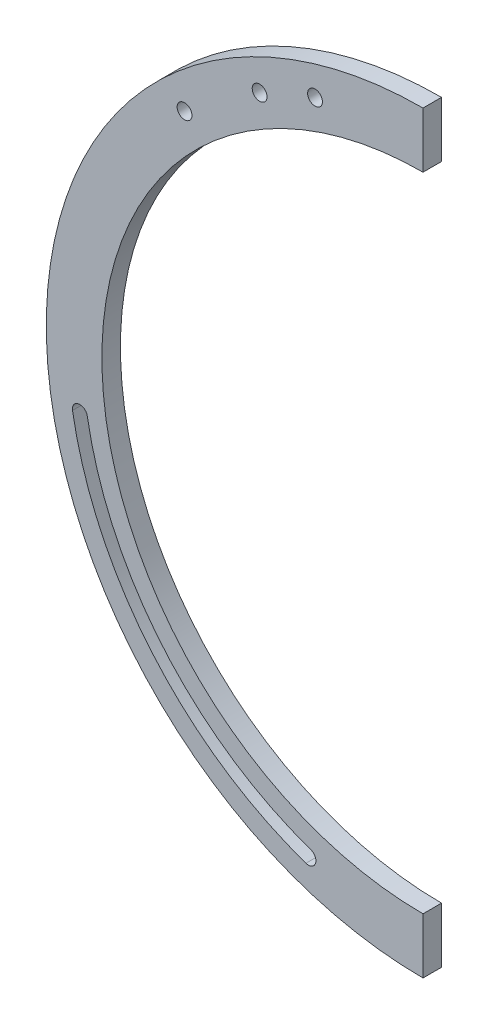
from build123d import *

# Parameters (mm, degrees)
SKETCH1_R               = 203.294925519
SKETCH1_R_2             = 173.294925519
BOSS_EXTRUDE1_DEPTH     = 10
CUT_EXTRUDE1_START      = -185
CUT_EXTRUDE1_DEPTH      = 185
CUT_EXTRUDE2_DEPTH      = 185
CUT_EXTRUDE3_DEPTH      = 484.877792972
CUT_EXTRUDE3_DEPTH_BACK = 484.877792972
SKETCH5_R               = 4


with BuildPart() as part:
    # Sketch1 → Boss-Extrude1 (new body)
    with BuildSketch(Plane.XY):
        with Locations((291.585214163, 182.730697222)):
            Circle(SKETCH1_R)
        with Locations((291.585214163, 182.730697222)):
            Circle(SKETCH1_R_2, mode=Mode.SUBTRACT)
    extrude(amount=-BOSS_EXTRUDE1_DEPTH)

    # Sketch2 → Cut-Extrude1 (cut)
    with BuildSketch(Plane(origin=(0, 0, -10), x_dir=(-1, 0, 0), z_dir=(0, 0, -1)).offset(CUT_EXTRUDE1_START)):
        with BuildLine():
            Line((-291.585214163, 9.435771703), (-291.585214163, -33.905509081))
            ThreePointArc((-291.585214163, -33.905509081), (-508.221420466, 182.730697222), (-291.585214163, 399.366903525))
            Line((-291.585214163, 399.366903525), (-291.585214163, 356.025622742))
            ThreePointArc((-291.585214163, 356.025622742), (-464.880139683, 182.730697222), (-291.585214163, 9.435771703))
        make_face()
    extrude(amount=CUT_EXTRUDE1_DEPTH, mode=Mode.SUBTRACT)

    # Sketch3 → Cut-Extrude2 (cut)
    with BuildSketch(Plane(origin=(0, 0, -10), x_dir=(-1, 0, 0), z_dir=(0, 0, -1))):
        with BuildLine():
            ThreePointArc((-228.398227799, 1.480100191), (-145.149611461, 58.629978323), (-102.426094867, 150.123922508))
            ThreePointArc((-102.426094867, 150.123922508), (-105.727828311, 154.801028245), (-110.404934048, 151.499294801))
            ThreePointArc((-110.404934048, 151.499294801), (-151.326348425, 63.864617192), (-231.063490803, 9.125353407))
            ThreePointArc((-231.063490803, 9.125353407), (-233.553485909, 3.970095297), (-228.398227799, 1.480100191))
        make_face()
    extrude(amount=-CUT_EXTRUDE2_DEPTH, mode=Mode.SUBTRACT)

    # Sketch5 → Cut-Extrude3 (cut, two sides: drawn at the far end of the back side and taken through both)
    with BuildSketch(Plane.XY.offset(-CUT_EXTRUDE3_DEPTH_BACK)):
        with Locations((233.317748738, 361.783430933)):
            Circle(SKETCH5_R)
        with Locations((203.411601384, 349.104953001)):
            Circle(SKETCH5_R)
        with Locations((162.898022452, 320.188274917)):
            Circle(SKETCH5_R)
    extrude(amount=CUT_EXTRUDE3_DEPTH + CUT_EXTRUDE3_DEPTH_BACK, mode=Mode.SUBTRACT)


solid = part.part
